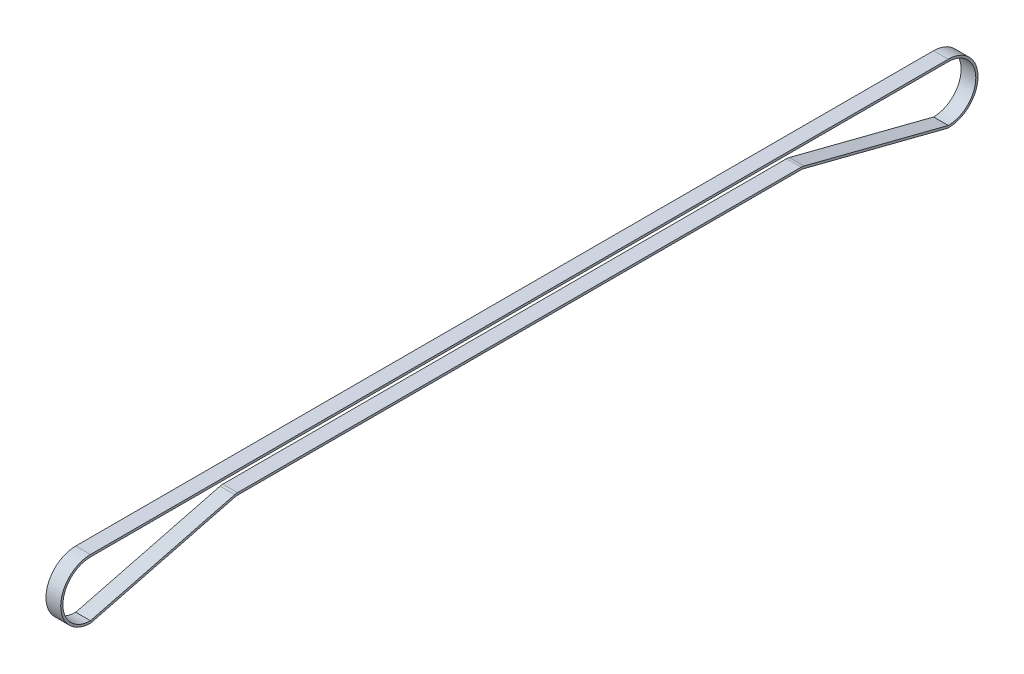
SolidWorks part; units mm, degrees
material "聚脂树脂"
ref_plane "前视基准面" through (0, 0, 0) normal (0, 0, 1) x (1, 0, 0)
ref_plane "上视基准面" through (0, 0, 0) normal (0, 1, 0) x (1, 0, 0)
ref_plane "右视基准面" through (0, 0, 0) normal (1, 0, 0) x (0, 0, -1)
sketch "草图2" plane through (0, 0, 0) normal (1, 0, 0) x (0, 0, -1)
  line L0 (0, 57.295) -> (-1750, 57.295)
  line L1 (0, -57.295) -> (-294.5304, 18.3042)
  line L2 (-1450, 18.995) -> (-300, 18.995)
  line L3 (-1455.4696, 18.3042) -> (-1750, -57.295)
  line L4 (-875, 18.995) -> (-875, -57.295) construction
  line L6 (-1750, -57.295) -> (0, -57.295) construction
  arc A0 (0, -57.295) -> (0, 57.295) centre (0, 0) ccw
  arc A1 (-1750, 57.295) -> (-1750, -57.295) centre (-1750, 0) ccw
  arc A2 (-1450, 18.995) -> (-1455.4696, 18.3042) centre (-1450, -3.005) ccw
  arc A3 (-300, 18.995) -> (-294.5304, 18.3042) centre (-300, -3.005) cw
  dimension "D1" = 44
  dimension "D2" = 114.59
  dimension "D3" = 54.29
  dimension "D4" = 300
  dimension "D7" = 1750
extrude "拉伸-薄壁1" add sketch "草图2" along normal mid plane 30 thin
